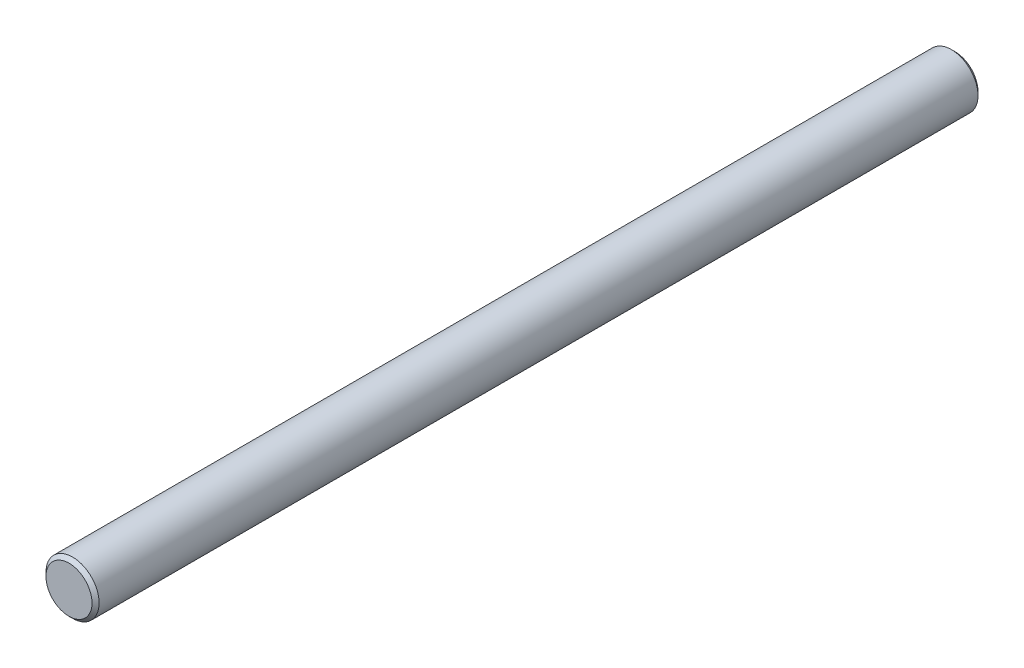
from build123d import *

# Parameters (mm, degrees)
SKETCH1_R           = 0.75
BOSS_EXTRUDE1_DEPTH = 12.5
CHAMFER1_SIZE       = 0.1


with BuildPart() as part:
    # Sketch1 → Boss-Extrude1 (new, symmetric)
    with BuildSketch(Plane.XY):
        Circle(SKETCH1_R)
    extrude(amount=BOSS_EXTRUDE1_DEPTH, both=True)

    # Chamfer1
    chamfer1_edges = [part.edges().sort_by_distance(p)[0] for p in [
        (-0.75, 0, -12.5),
        (-0.75, 0, 12.5),
    ]]
    chamfer(chamfer1_edges, length=CHAMFER1_SIZE)


solid = part.part
